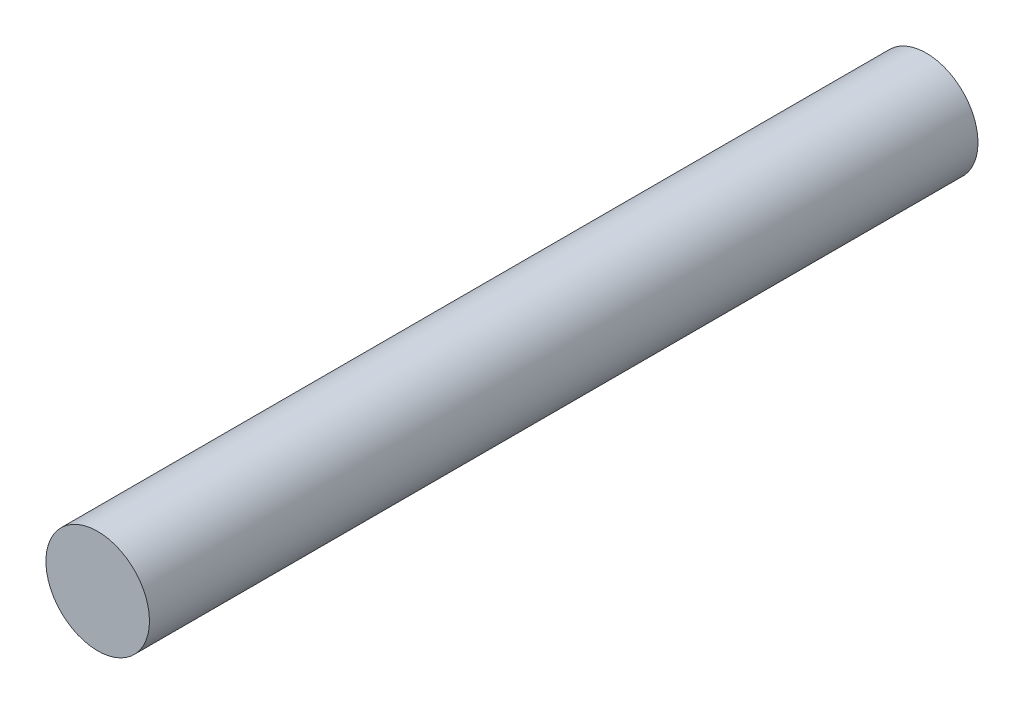
SolidWorks part; units mm, degrees
ref_plane "Front Plane" through (0, 0, 0) normal (0, 0, 1) x (1, 0, 0)
ref_plane "Top Plane" through (0, 0, 0) normal (0, 1, 0) x (1, 0, 0)
ref_plane "Right Plane" through (0, 0, 0) normal (1, 0, 0) x (0, 0, -1)
other "Configuration Table"
sketch "Sketch1" plane through (0, 0, 0) normal (0, 0, 1) x (1, 0, 0)
  circle A0 centre (0, 0) radius 2.5
  dimension "D1" = 5
extrude "Boss-Extrude1" add sketch "Sketch1" along normal blind 40
